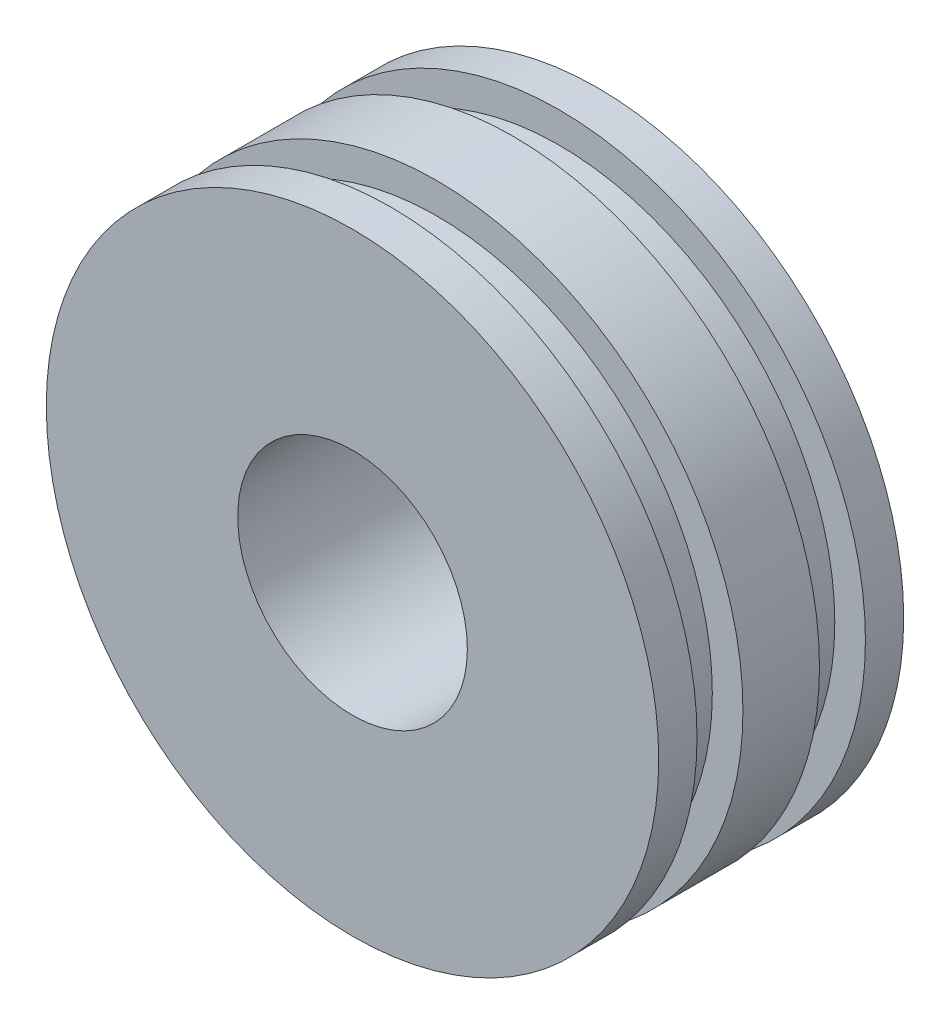
SolidWorks part; units mm, degrees
ref_plane "前视基准面" through (0, 0, 0) normal (0, 0, 1) x (1, 0, 0)
ref_plane "上视基准面" through (0, 0, 0) normal (0, 1, 0) x (1, 0, 0)
ref_plane "右视基准面" through (0, 0, 0) normal (1, 0, 0) x (0, 0, -1)
other "Configuration Table"
sketch "草图1" plane through (0, 0, 0) normal (0, 0, 1) x (1, 0, 0)
  circle A0 centre (0, 0) radius 37.5
  circle A1 centre (0, 0) radius 100
  dimension "D1" = 75
  dimension "D2" = 200
extrude "凸台-拉伸1" add sketch "草图1" along normal mid plane 80
ref_plane "基准面1" through (0, 0, 20) normal (0, 0, 1) x (1, 0, 0)
sketch "草图2" plane through (0, 0, 20) normal (0, 0, 1) x (1, 0, 0)
  circle A0 centre (0, 0) radius 100 construction
  circle A1 centre (0, 0) radius 100
  circle A2 centre (0, 0) radius 90
  dimension "D1" = 180
extrude "切除-拉伸1" cut sketch "草图2" against normal mid plane 15
mirror "镜向1" about plane through (0, 0, 0) normal (0, 0, 1) of "切除-拉伸1"
